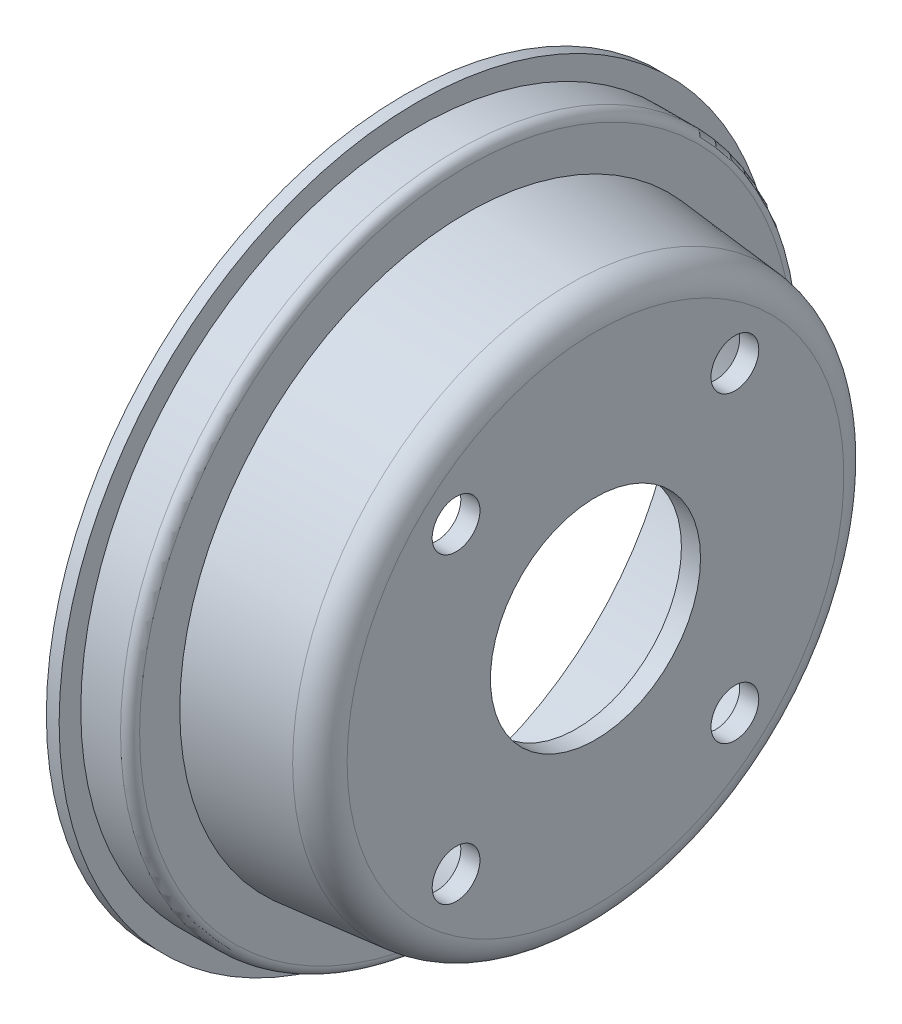
SolidWorks part; units mm, degrees
ref_plane "Front Plane" through (0, 0, 0) normal (0, 0, 1) x (1, 0, 0)
ref_plane "Top Plane" through (0, 0, 0) normal (0, 1, 0) x (1, 0, 0)
ref_plane "Right Plane" through (0, 0, 0) normal (1, 0, 0) x (0, 0, -1)
sketch "Sketch1" plane through (0, 0, 0) normal (0, 0, 1) x (1, 0, 0)
  line L0 (-61.4974, 25.5648) -> (-16.9123, 25.5648) construction
  line L1 (-61.4974, 54.2074) -> (-61.4974, 63.0648)
  line L2 (-61.4974, 63.0648) -> (-60.1579, 63.0648)
  line L3 (-60.1579, 63.0648) -> (-60.1579, 60.7984)
  line L4 (-60.1579, 60.7984) -> (-54.9974, 60.7984)
  line L5 (-54.9974, 60.7984) -> (-54.9974, 55.5937)
  line L6 (-54.9974, 55.5937) -> (-41.4974, 54.3)
  line L7 (-41.4974, 54.3) -> (-41.4974, 25.5648)
  line L8 (-61.4974, 54.2074) -> (-43.4974, 52.4825)
  line L9 (-43.4974, 52.4825) -> (-43.4974, 25.5648)
  line L10 (-41.4974, 25.5648) -> (-43.4974, 25.5648)
  dimension "D1" = 20
  dimension "D2" = 2
  dimension "D3" = 2
  dimension "D4" = 37.5
  dimension "D5" = 20
revolve "Revolve1" add sketch "Sketch1" angle 360 about L0
sketch "Sketch2" plane through (-41.4974, 0, 0) normal (1, 0, 0) x (0, 0, -1)
  line L0 (0, 54.3) -> (0, -3.1703) construction
  line L1 (-28.7351, 25.5648) -> (28.7351, 25.5648) construction
  circle A0 centre (0, 25.5648) radius 11
  circle A1 centre (0, 25.5648) radius 28.7351 construction
  circle A2 centre (-14.5987, 41.4201) radius 2.5
  circle A3 centre (14.5987, 41.4201) radius 2.5
  circle A4 centre (14.5987, 9.7095) radius 2.5
  circle A5 centre (-14.5987, 9.7095) radius 2.5
  dimension "D1" = 22
  dimension "D2" = 5
extrude "Cut-Extrude1" cut sketch "Sketch2" against normal blind 10
fillet "Fillet1" radius 3 1 edges at (-41.4974, 25.5648, 28.7351)
fillet "Fillet2" radius 1 1 edges at (-54.9974, 25.5648, 35.2335)
